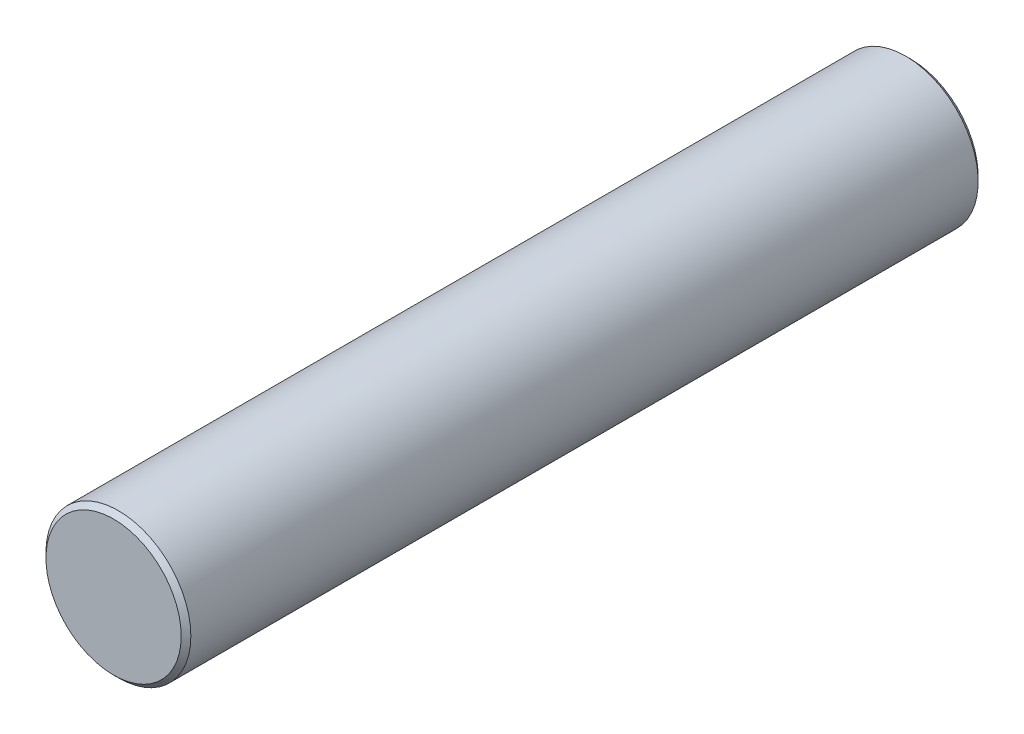
from build123d import *

# Parameters (mm, degrees)
SKETCH1_R           = 3
BOSS_EXTRUDE1_DEPTH = 16.5
CHAMFER1_SIZE       = 0.2
SKETCH2_W           = 0.5
SKETCH2_H           = 10
CUT_EXTRUDE1_DEPTH  = 15


with BuildPart() as part:
    # Sketch1 → Boss-Extrude1 (new, symmetric)
    with BuildSketch(Plane.XY):
        Circle(SKETCH1_R)
    extrude(amount=BOSS_EXTRUDE1_DEPTH, both=True)

    # Chamfer1
    chamfer1_edges = [part.edges().sort_by_distance(p)[0] for p in [
        (-3, 0, -16.5),
        (-3, 0, 16.5),
    ]]
    chamfer(chamfer1_edges, length=CHAMFER1_SIZE)

    # Sketch2 → Cut-Extrude1 (cut, symmetric)
    with BuildSketch(Plane(origin=(0, 0, 0), x_dir=(1, 0, 0), z_dir=(0, 1, 0))):
        with Locations((-2.75, 11.5)):
            Rectangle(SKETCH2_W, SKETCH2_H)
    extrude(amount=CUT_EXTRUDE1_DEPTH, both=True, mode=Mode.SUBTRACT)


solid = part.part
